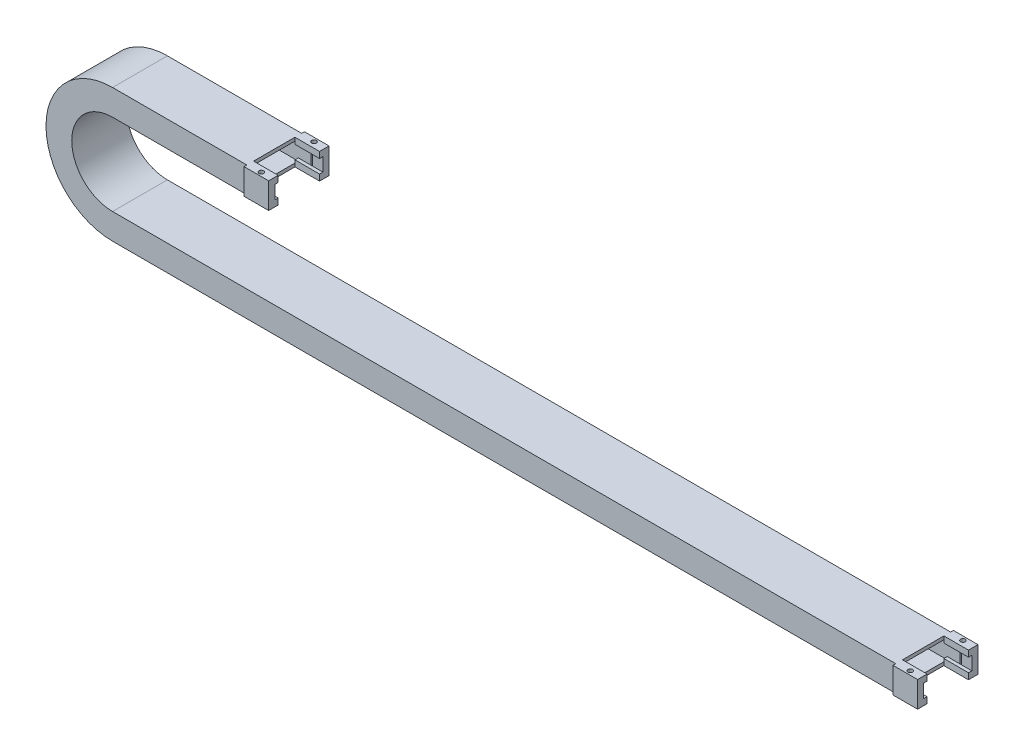
from build123d import *

# Parameters (mm, degrees)
SKETCH_2_W                  = 49
SKETCH_2_H                  = 23
SHELL_1_T                   = -3
SKETCH_11_W                 = 54
SKETCH_11_H                 = 23
SKETCH_11_W_2               = 43
SKETCH_11_H_2               = 12
EXTRUDE_1_DEPTH             = 22
SKETCH_12_W                 = 23.011901601
SKETCH_12_H                 = 37
CUT_EXTRUDE_9_DEPTH         = 767.019092451
HOLE_WIZARD_4_2_4_2_1_D     = 4.2
SKETCH_15_W                 = 54
SKETCH_15_H                 = 23
SKETCH_15_W_2               = 43
SKETCH_15_H_2               = 12
EXTRUDE_2_DEPTH             = 22
SKETCH_16_W                 = 45.795478168
SKETCH_16_H                 = 37
CUT_EXTRUDE_10_DEPTH        = 49
HOLE_WIZARD_4_2_4_2_2_D     = 4.2
HOLE_WIZARD_4_2_4_2_2_DEPTH = 50
HOLE_WIZARD_4_2_4_2_2_TIP   = 1.2618073


with BuildPart() as part:
    # 扫描1: sweep along a path in 草图1
    with BuildLine(Plane.XY) as sweep_1_path:
        Line((0, 0), (-700, 0))
        ThreePointArc((-700, 0), (-748, 48), (-700, 96))
        Line((-700, 96), (-580, 96))
    # 草图2 → 扫描1 (sweep)
    with BuildSketch(Plane(origin=(0, 0, 0), x_dir=(0, 0, -1), z_dir=(1, 0, 0))):
        Rectangle(SKETCH_2_W, SKETCH_2_H)
    sweep(path=sweep_1_path.line)

    # 抽壳1
    shell_1_openings = [part.faces().sort_by_distance(p)[0] for p in [
        (-580, 96, 0),
        (0, 0, 0),
    ]]
    offset(amount=SHELL_1_T, openings=shell_1_openings, kind=Kind.INTERSECTION)

    # 草图11 → 凸台-拉伸1 (add)
    with BuildSketch(Plane(origin=(0, 0, 0), x_dir=(0, 0, -1), z_dir=(1, 0, 0))):
        Rectangle(SKETCH_11_W, SKETCH_11_H)
        Rectangle(SKETCH_11_W_2, SKETCH_11_H_2, mode=Mode.SUBTRACT)
    extrude(amount=EXTRUDE_1_DEPTH)

    # 草图12 → 切除-拉伸9 (cut, through all)
    with BuildSketch(Plane(origin=(0, 11.5, 0), x_dir=(1, 0, 0), z_dir=(0, 1, 0))):
        with Locations((11.505950801, 0)):
            Rectangle(SKETCH_12_W, SKETCH_12_H)
    extrude(amount=-CUT_EXTRUDE_9_DEPTH, mode=Mode.SUBTRACT)

    # Ø4.2 (4.2) 直径孔1 (through all)
    with Locations(Plane(origin=(0, 11.5, 0), x_dir=(1, 0, 0), z_dir=(0, 1, 0))):
        with Locations((12, 23.5), (12, -23.5)):
            Hole(HOLE_WIZARD_4_2_4_2_1_D / 2)

    # 草图15 → 凸台-拉伸2 (add)
    with BuildSketch(Plane(origin=(-580, 0, 0), x_dir=(0, 0, -1), z_dir=(1, 0, 0))):
        with Locations((0, 96)):
            Rectangle(SKETCH_15_W, SKETCH_15_H)
        with Locations((0, 96)):
            Rectangle(SKETCH_15_W_2, SKETCH_15_H_2, mode=Mode.SUBTRACT)
    extrude(amount=EXTRUDE_2_DEPTH)

    # 草图16 → 切除-拉伸10 (cut)
    with BuildSketch(Plane(origin=(0, 107.5, 0), x_dir=(1, 0, 0), z_dir=(0, 1, 0))):
        with Locations((-557.102260916, 0)):
            Rectangle(SKETCH_16_W, SKETCH_16_H)
    extrude(amount=-CUT_EXTRUDE_10_DEPTH, mode=Mode.SUBTRACT)

    # Ø4.2 (4.2) 直径孔2
    with Locations(Plane(origin=(0, 107.5, 0), x_dir=(1, 0, 0), z_dir=(0, 1, 0))):
        with Locations((-568, 23.5), (-568, -23.5)):
            Hole(HOLE_WIZARD_4_2_4_2_2_D / 2, depth=HOLE_WIZARD_4_2_4_2_2_DEPTH)
            with Locations((0, 0, -(HOLE_WIZARD_4_2_4_2_2_DEPTH + HOLE_WIZARD_4_2_4_2_2_TIP / 2))):  # 118° drill point
                Cone(0, HOLE_WIZARD_4_2_4_2_2_D / 2, HOLE_WIZARD_4_2_4_2_2_TIP, mode=Mode.SUBTRACT)


solid = part.part
